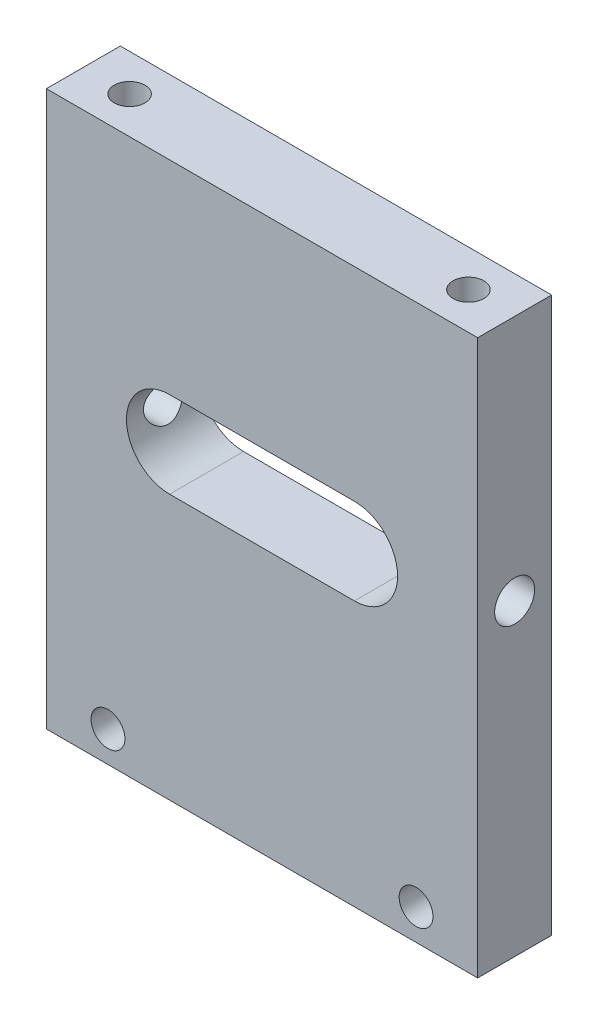
from build123d import *

# Parameters (mm, degrees)
SKETCH_1_W             = 70
SKETCH_1_H             = 90
EXTRUDE_1_DEPTH        = 12
CUT_EXTRUDE_1_DEPTH    = 115.647285184
SKETCH_4_R             = 3.25
CUT_EXTRUDE_2_DEPTH    = 115.647285184
HOLE_WIZARD_M6_1_D     = 5
HOLE_WIZARD_M6_1_DEPTH = 17
HOLE_WIZARD_M6_1_TIP   = 1.502151548
SKETCH_11_R            = 2.75
CUT_EXTRUDE_3_DEPTH    = 115.647285255


with BuildPart() as part:
    # 草图1 → 凸台-拉伸1 (new body)
    with BuildSketch(Plane.XY):
        with Locations((35, -45)):
            Rectangle(SKETCH_1_W, SKETCH_1_H)
    extrude(amount=EXTRUDE_1_DEPTH)

    # 草图2 → 切除-拉伸1 (cut, through all)
    with BuildSketch(Plane.XY.offset(12)):
        with BuildLine():
            Line((20, -33), (50, -33))
            ThreePointArc((50, -33), (57, -40), (50, -47))
            Line((50, -47), (20, -47))
            ThreePointArc((20, -47), (13, -40), (20, -33))
        make_face()
    extrude(amount=-CUT_EXTRUDE_1_DEPTH, mode=Mode.SUBTRACT)

    # 草图4 → 切除-拉伸2 (cut, through all)
    with BuildSketch(Plane(origin=(70, 0, 0), x_dir=(0, 0, -1), z_dir=(1, 0, 0))):
        with Locations((-6, -40)):
            Circle(SKETCH_4_R)
    extrude(amount=-CUT_EXTRUDE_2_DEPTH, mode=Mode.SUBTRACT)

    # M6 螺纹孔1
    with Locations(Plane(origin=(0, 0, 0), x_dir=(1, 0, 0), z_dir=(0, 1, 0))):
        with Locations((62.5, -6), (7.5, -6)):
            Hole(HOLE_WIZARD_M6_1_D / 2, depth=HOLE_WIZARD_M6_1_DEPTH)
            with Locations((0, 0, -(HOLE_WIZARD_M6_1_DEPTH + HOLE_WIZARD_M6_1_TIP / 2))):  # 118° drill point
                Cone(0, HOLE_WIZARD_M6_1_D / 2, HOLE_WIZARD_M6_1_TIP, mode=Mode.SUBTRACT)

    # 草图11 → 切除-拉伸3 (cut, through all)
    with BuildSketch(Plane.XY.offset(12)):
        with Locations((10, -85)):
            Circle(SKETCH_11_R)
        with Locations((60, -85)):
            Circle(SKETCH_11_R)
    extrude(amount=-CUT_EXTRUDE_3_DEPTH, mode=Mode.SUBTRACT)


solid = part.part
